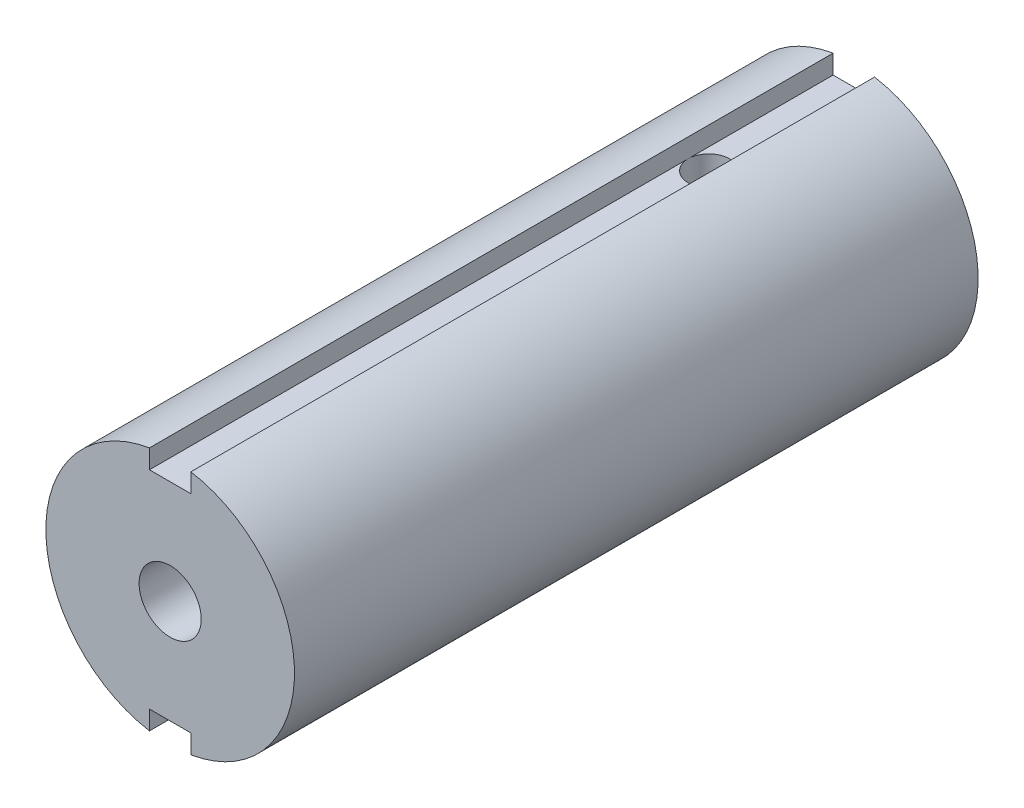
from build123d import *

# Parameters (mm, degrees)
SKETCH1_R           = 6
BOSS_EXTRUDE1_DEPTH = 33
SKETCH2_W           = 2
SKETCH2_H           = 2
CUT_EXTRUDE1_DEPTH  = 33
SKETCH3_R           = 1.5
CUT_EXTRUDE2_DEPTH  = 23
SKETCH4_R           = 1
CUT_EXTRUDE3_DEPTH  = 7
SKETCH5_R           = 3.5
CUT_EXTRUDE4_DEPTH  = 2
SKETCH6_R           = 3.4
BOSS_EXTRUDE2_DEPTH = 2


with BuildPart() as part:
    # Sketch1 → Boss-Extrude1 (new body)
    with BuildSketch(Plane.XY):
        Circle(SKETCH1_R)
    extrude(amount=BOSS_EXTRUDE1_DEPTH)

    # Sketch2 → Cut-Extrude1 (cut)
    with BuildSketch(Plane.XY.offset(33)):
        with Locations((0, 6)):
            Rectangle(SKETCH2_W, SKETCH2_H)
    cut_extrude1 = extrude(amount=-CUT_EXTRUDE1_DEPTH, mode=Mode.SUBTRACT)

    # Mirror1: Cut-Extrude1 across plane
    add(cut_extrude1.mirror(Plane.ZX), mode=Mode.SUBTRACT)

    # Sketch3 → Cut-Extrude2 (cut)
    with BuildSketch(Plane.XY.offset(33)):
        Circle(SKETCH3_R)
    extrude(amount=-CUT_EXTRUDE2_DEPTH, mode=Mode.SUBTRACT)

    # Sketch4 → Cut-Extrude3 (cut)
    with BuildSketch(Plane(origin=(0, 5, 0), x_dir=(1, 0, 0), z_dir=(0, 1, 0))):
        with Locations(Location((0, -7, 0), (0, 0, 270))):
            Circle(SKETCH4_R)
    extrude(amount=-CUT_EXTRUDE3_DEPTH, mode=Mode.SUBTRACT)

    # Sketch5 → Cut-Extrude4 (cut)
    with BuildSketch(Plane(origin=(0, 0, 0), x_dir=(-1, 0, 0), z_dir=(0, 0, -1))):
        Circle(SKETCH5_R)
    extrude(amount=-CUT_EXTRUDE4_DEPTH, mode=Mode.SUBTRACT)

    # Sketch6 → Boss-Extrude2 (add)
    with BuildSketch(Plane(origin=(0, 0, 2), x_dir=(-1, 0, 0), z_dir=(0, 0, -1))):
        with Locations(Location((0, 0, 0), (0, 0, 180))):
            Circle(SKETCH6_R)
    extrude(amount=BOSS_EXTRUDE2_DEPTH)


solid = part.part
